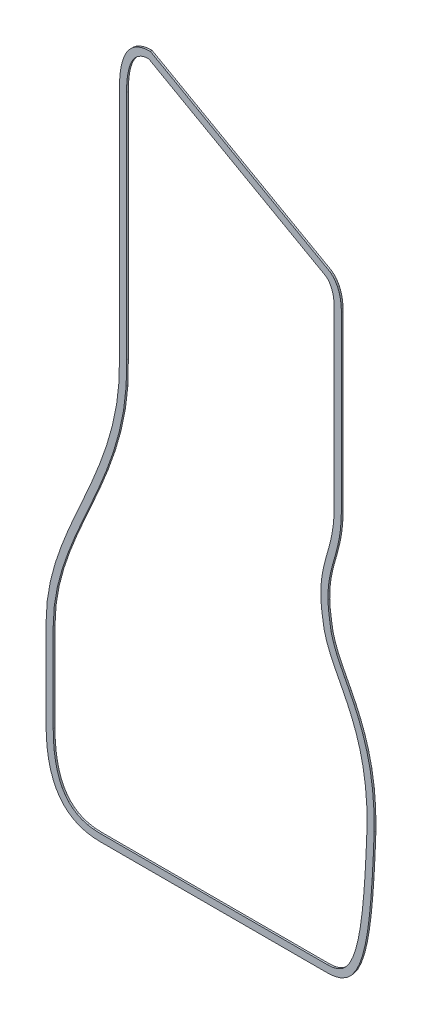
SolidWorks part; units mm, degrees
ref_plane "前视基准面" through (0, 0, 0) normal (0, 0, 1) x (1, 0, 0)
ref_plane "上视基准面" through (0, 0, 0) normal (0, 1, 0) x (1, 0, 0)
ref_plane "右视基准面" through (0, 0, 0) normal (1, 0, 0) x (0, 0, -1)
other "Configuration Table"
sketch "草图1" plane through (0, 0, 0) normal (0, 0, 1) x (1, 0, 0)
  line L0 (103, 235) -> (-24.8333, 235)
  line L1 (-24.8333, 235) -> (-152.6667, 235)
  line L2 (-152.6667, 235) -> (-280.5, 235)
  line L3 (-280.5, 235) -> (-293.0357, 235.6378)
  line L4 (-293.0357, 235.6378) -> (-304.6429, 237.551)
  line L5 (-304.6429, 237.551) -> (-315.3214, 240.7398)
  line L6 (-315.3214, 240.7398) -> (-325.0714, 245.2041)
  line L7 (-325.0714, 245.2041) -> (-333.8929, 250.9439)
  line L8 (-333.8929, 250.9439) -> (-341.7857, 257.9592)
  line L9 (-341.7857, 257.9592) -> (-348.75, 266.25)
  line L10 (-348.75, 266.25) -> (-354.7857, 275.8163)
  line L11 (-354.7857, 275.8163) -> (-359.8929, 286.6582)
  line L12 (-359.8929, 286.6582) -> (-364.0714, 298.7755)
  line L13 (-364.0714, 298.7755) -> (-367.3214, 312.1684)
  line L14 (-367.3214, 312.1684) -> (-369.6429, 326.8367)
  line L15 (-369.6429, 326.8367) -> (-371.0357, 342.7806)
  line L16 (-371.0357, 342.7806) -> (-371.5, 360)
  line L17 (-371.5, 360) -> (-371.5, 410)
  line L18 (-371.5, 410) -> (-371.5, 460)
  line L19 (-371.5, 460) -> (-371.5, 510)
  line L20 (-371.5, 510) -> (-369.6073, 541.7165)
  line L21 (-369.6073, 541.7165) -> (-364.3178, 572.7114)
  line L22 (-364.3178, 572.7114) -> (-356.2141, 603.1815)
  line L23 (-356.2141, 603.1815) -> (-345.879, 633.3236)
  line L24 (-345.879, 633.3236) -> (-333.8952, 663.3345)
  line L25 (-333.8952, 663.3345) -> (-320.8455, 693.4111)
  line L26 (-320.8455, 693.4111) -> (-307.3125, 723.75)
  line L27 (-307.3125, 723.75) -> (-293.879, 754.5481)
  line L28 (-293.879, 754.5481) -> (-281.1277, 786.0022)
  line L29 (-281.1277, 786.0022) -> (-269.6414, 818.309)
  line L30 (-269.6414, 818.309) -> (-260.0027, 851.6655)
  line L31 (-260.0027, 851.6655) -> (-252.7945, 886.2682)
  line L32 (-252.7945, 886.2682) -> (-248.5993, 922.3141)
  line L33 (-248.5993, 922.3141) -> (-248, 960)
  line L34 (-248, 960) -> (-248, 1090)
  line L35 (-248, 1090) -> (-248, 1220)
  line L36 (-248, 1220) -> (-248, 1350)
  line L37 (-248, 1350) -> (-247.7347, 1361.0204)
  line L38 (-247.7347, 1361.0204) -> (-246.9388, 1371.2245)
  line L39 (-246.9388, 1371.2245) -> (-245.6122, 1380.6122)
  line L40 (-245.6122, 1380.6122) -> (-243.7551, 1389.1837)
  line L41 (-243.7551, 1389.1837) -> (-241.3673, 1396.9388)
  line L42 (-241.3673, 1396.9388) -> (-238.449, 1403.8776)
  line L43 (-238.449, 1403.8776) -> (-235, 1410)
  line L44 (-235, 1410) -> (-231.0204, 1415.3061)
  line L45 (-231.0204, 1415.3061) -> (-226.5102, 1419.7959)
  line L46 (-226.5102, 1419.7959) -> (-221.4694, 1423.4694)
  line L47 (-221.4694, 1423.4694) -> (-215.898, 1426.3265)
  line L48 (-215.898, 1426.3265) -> (-209.7959, 1428.3673)
  line L49 (-209.7959, 1428.3673) -> (-203.1633, 1429.5918)
  line L50 (-203.1633, 1429.5918) -> (-196, 1430)
  line L51 (-196, 1430) -> (-95.25, 1373.3333)
  line L52 (-95.25, 1373.3333) -> (5.5, 1316.6667)
  line L53 (5.5, 1316.6667) -> (106.25, 1260)
  line L54 (106.25, 1260) -> (108.9362, 1257.8878)
  line L55 (108.9362, 1257.8878) -> (111.4235, 1255.551)
  line L56 (111.4235, 1255.551) -> (113.7117, 1252.9898)
  line L57 (113.7117, 1252.9898) -> (115.801, 1250.2041)
  line L58 (115.801, 1250.2041) -> (117.6913, 1247.1939)
  line L59 (117.6913, 1247.1939) -> (119.3827, 1243.9592)
  line L60 (119.3827, 1243.9592) -> (120.875, 1240.5)
  line L61 (120.875, 1240.5) -> (122.1684, 1236.8163)
  line L62 (122.1684, 1236.8163) -> (123.2628, 1232.9082)
  line L63 (123.2628, 1232.9082) -> (124.1582, 1228.7755)
  line L64 (124.1582, 1228.7755) -> (124.8546, 1224.4184)
  line L65 (124.8546, 1224.4184) -> (125.352, 1219.8367)
  line L66 (125.352, 1219.8367) -> (125.6505, 1215.0306)
  line L67 (125.6505, 1215.0306) -> (125.75, 1210)
  line L68 (125.75, 1210) -> (125.75, 1113.3333)
  line L69 (125.75, 1113.3333) -> (125.75, 1016.6667)
  line L70 (125.75, 1016.6667) -> (125.75, 920)
  line L71 (125.75, 920) -> (125.281, 904.7303)
  line L72 (125.281, 904.7303) -> (123.9876, 890.9038)
  line L73 (123.9876, 890.9038) -> (122.0405, 878.2799)
  line L74 (122.0405, 878.2799) -> (119.6101, 866.6181)
  line L75 (119.6101, 866.6181) -> (116.867, 855.6778)
  line L76 (116.867, 855.6778) -> (113.9818, 845.2187)
  line L77 (113.9818, 845.2187) -> (111.125, 835)
  line L78 (111.125, 835) -> (108.4672, 824.7813)
  line L79 (108.4672, 824.7813) -> (106.1789, 814.3222)
  line L80 (106.1789, 814.3222) -> (104.4308, 803.3819)
  line L81 (104.4308, 803.3819) -> (103.3932, 791.7201)
  line L82 (103.3932, 791.7201) -> (103.2369, 779.0962)
  line L83 (103.2369, 779.0962) -> (104.1323, 765.2697)
  line L84 (104.1323, 765.2697) -> (106.25, 750)
  line L85 (106.25, 750) -> (108.5868, 735.4045)
  line L86 (108.5868, 735.4045) -> (112.6079, 721.3994)
  line L87 (112.6079, 721.3994) -> (118.0076, 707.6567)
  line L88 (118.0076, 707.6567) -> (124.4803, 693.8484)
  line L89 (124.4803, 693.8484) -> (131.7206, 679.6465)
  line L90 (131.7206, 679.6465) -> (139.4227, 664.723)
  line L91 (139.4227, 664.723) -> (147.2812, 648.75)
  line L92 (147.2812, 648.75) -> (154.9905, 631.3994)
  line L93 (154.9905, 631.3994) -> (162.245, 612.3433)
  line L94 (162.245, 612.3433) -> (168.7391, 591.2536)
  line L95 (168.7391, 591.2536) -> (174.1672, 567.8025)
  line L96 (174.1672, 567.8025) -> (178.2238, 541.6618)
  line L97 (178.2238, 541.6618) -> (180.6032, 512.5036)
  line L98 (180.6032, 512.5036) -> (181, 480)
  line L99 (181, 480) -> (179.4934, 443.1706)
  line L100 (179.4934, 443.1706) -> (177.7026, 409.7522)
  line L101 (177.7026, 409.7522) -> (175.5423, 379.6356)
  line L102 (175.5423, 379.6356) -> (172.9271, 352.7114)
  line L103 (172.9271, 352.7114) -> (169.7719, 328.8703)
  line L104 (169.7719, 328.8703) -> (165.9913, 308.0029)
  line L105 (165.9913, 308.0029) -> (161.5, 290)
  line L106 (161.5, 290) -> (156.2128, 274.7522)
  line L107 (156.2128, 274.7522) -> (150.0445, 262.1501)
  line L108 (150.0445, 262.1501) -> (142.9096, 252.0845)
  line L109 (142.9096, 252.0845) -> (134.723, 244.4461)
  line L110 (134.723, 244.4461) -> (125.3994, 239.1254)
  line L111 (125.3994, 239.1254) -> (114.8535, 236.0131)
  line L112 (114.8535, 236.0131) -> (103, 235)
  line L113 (102.4881, 247) -> (-280.1949, 247)
  line L114 (-280.1949, 247) -> (-291.751, 247.5879)
  line L115 (-291.751, 247.5879) -> (-301.9394, 249.2673)
  line L116 (-301.9394, 249.2673) -> (-311.0863, 251.9987)
  line L117 (-311.0863, 251.9987) -> (-319.2698, 255.7457)
  line L118 (-319.2698, 255.7457) -> (-326.5937, 260.5112)
  line L119 (-326.5937, 260.5112) -> (-333.1599, 266.3473)
  line L120 (-333.1599, 266.3473) -> (-339.0366, 273.3434)
  line L121 (-339.0366, 273.3434) -> (-344.2438, 281.5965)
  line L122 (-344.2438, 281.5965) -> (-348.7602, 291.1843)
  line L123 (-348.7602, 291.1843) -> (-352.543, 302.1539)
  line L124 (-352.543, 302.1539) -> (-355.5451, 314.5251)
  line L125 (-355.5451, 314.5251) -> (-357.7249, 328.2986)
  line L126 (-357.7249, 328.2986) -> (-359.0498, 343.4651)
  line L127 (-359.0498, 343.4651) -> (-359.5, 360.1617)
  line L128 (-359.5, 360.1617) -> (-359.5, 509.6423)
  line L129 (-359.5, 509.6423) -> (-357.6678, 540.3456)
  line L130 (-357.6678, 540.3456) -> (-352.5806, 570.1546)
  line L131 (-352.5806, 570.1546) -> (-344.7258, 599.689)
  line L132 (-344.7258, 599.689) -> (-334.6243, 629.1499)
  line L133 (-334.6243, 629.1499) -> (-322.8164, 658.7203)
  line L134 (-322.8164, 658.7203) -> (-309.8614, 688.5785)
  line L135 (-309.8614, 688.5785) -> (-296.3533, 718.8616)
  line L136 (-296.3533, 718.8616) -> (-296.3133, 718.9524)
  line L137 (-296.3133, 718.9524) -> (-282.8798, 749.7505)
  line L138 (-282.8798, 749.7505) -> (-282.7581, 750.0398)
  line L139 (-282.7581, 750.0398) -> (-270.0068, 781.4938)
  line L140 (-270.0068, 781.4938) -> (-269.8211, 781.9822)
  line L141 (-269.8211, 781.9822) -> (-258.3348, 814.2891)
  line L142 (-258.3348, 814.2891) -> (-258.113, 814.9778)
  line L143 (-258.113, 814.9778) -> (-248.4744, 848.3342)
  line L144 (-248.4744, 848.3342) -> (-248.2549, 849.2182)
  line L145 (-248.2549, 849.2182) -> (-241.0467, 883.821)
  line L146 (-241.0467, 883.821) -> (-240.8749, 884.881)
  line L147 (-240.8749, 884.881) -> (-236.6798, 920.9269)
  line L148 (-236.6798, 920.9269) -> (-236.6008, 922.1233)
  line L149 (-236.6008, 922.1233) -> (-236.0015, 959.8092)
  line L150 (-236.0015, 959.8092) -> (-236, 960)
  line L151 (-236, 960) -> (-236, 1349.8556)
  line L152 (-236, 1349.8556) -> (-235.7459, 1360.409)
  line L153 (-235.7459, 1360.409) -> (-235.0043, 1369.9171)
  line L154 (-235.0043, 1369.9171) -> (-233.7916, 1378.4994)
  line L155 (-233.7916, 1378.4994) -> (-232.1357, 1386.142)
  line L156 (-232.1357, 1386.142) -> (-230.0744, 1392.8369)
  line L157 (-230.0744, 1392.8369) -> (-227.6551, 1398.5891)
  line L158 (-227.6551, 1398.5891) -> (-224.9296, 1403.4272)
  line L159 (-224.9296, 1403.4272) -> (-221.9403, 1407.4129)
  line L160 (-221.9403, 1407.4129) -> (-218.6976, 1410.6409)
  line L161 (-218.6976, 1410.6409) -> (-215.1595, 1413.2193)
  line L162 (-215.1595, 1413.2193) -> (-211.2304, 1415.2342)
  line L163 (-211.2304, 1415.2342) -> (-206.7888, 1416.7197)
  line L164 (-206.7888, 1416.7197) -> (-201.727, 1417.6542)
  line L165 (-201.727, 1417.6542) -> (-198.8226, 1417.8197)
  line L166 (-198.8226, 1417.8197) -> (-101.1327, 1362.8742)
  line L167 (-101.1327, 1362.8742) -> (99.5603, 1249.9947)
  line L168 (99.5603, 1249.9947) -> (101.1041, 1248.7808)
  line L169 (101.1041, 1248.7808) -> (102.8244, 1247.1646)
  line L170 (102.8244, 1247.1646) -> (104.4203, 1245.3783)
  line L171 (104.4203, 1245.3783) -> (105.9029, 1243.4016)
  line L172 (105.9029, 1243.4016) -> (107.2769, 1241.2136)
  line L173 (107.2769, 1241.2136) -> (108.5414, 1238.7952)
  line L174 (108.5414, 1238.7952) -> (109.6911, 1236.1303)
  line L175 (109.6911, 1236.1303) -> (110.7175, 1233.2069)
  line L176 (110.7175, 1233.2069) -> (111.6107, 1230.0172)
  line L177 (111.6107, 1230.0172) -> (112.3606, 1226.5563)
  line L178 (112.3606, 1226.5563) -> (112.9573, 1222.8227)
  line L179 (112.9573, 1222.8227) -> (113.3923, 1218.8167)
  line L180 (113.3923, 1218.8167) -> (113.6579, 1214.5399)
  line L181 (113.6579, 1214.5399) -> (113.75, 1209.8814)
  line L182 (113.75, 1209.8814) -> (113.75, 920.1843)
  line L183 (113.75, 920.1843) -> (113.2982, 905.4741)
  line L184 (113.2982, 905.4741) -> (112.0732, 892.3786)
  line L185 (112.0732, 892.3786) -> (110.2287, 880.4201)
  line L186 (110.2287, 880.4201) -> (107.9117, 869.3025)
  line L187 (107.9117, 869.3025) -> (105.2616, 858.733)
  line L188 (105.2616, 858.733) -> (102.4193, 848.4296)
  line L189 (102.4193, 848.4296) -> (99.5681, 838.2309)
  line L190 (99.5681, 838.2309) -> (99.5114, 838.0206)
  line L191 (99.5114, 838.0206) -> (96.8536, 827.802)
  line L192 (96.8536, 827.802) -> (96.7445, 827.346)
  line L193 (96.7445, 827.346) -> (94.4562, 816.8869)
  line L194 (94.4562, 816.8869) -> (94.3293, 816.2157)
  line L195 (94.3293, 816.2157) -> (92.5811, 805.2754)
  line L196 (92.5811, 805.2754) -> (92.478, 804.4453)
  line L197 (92.478, 804.4453) -> (91.4404, 792.7835)
  line L198 (91.4404, 792.7835) -> (91.3941, 791.8687)
  line L199 (91.3941, 791.8687) -> (91.2378, 779.2448)
  line L200 (91.2378, 779.2448) -> (91.262, 778.3207)
  line L201 (91.262, 778.3207) -> (92.1574, 764.4942)
  line L202 (92.1574, 764.4942) -> (92.2461, 763.6212)
  line L203 (92.2461, 763.6212) -> (94.3638, 748.3515)
  line L204 (94.3638, 748.3515) -> (94.4009, 748.1029)
  line L205 (94.4009, 748.1029) -> (96.7377, 733.5074)
  line L206 (96.7377, 733.5074) -> (97.0528, 732.093)
  line L207 (97.0528, 732.093) -> (101.0739, 718.0879)
  line L208 (101.0739, 718.0879) -> (101.4391, 717.011)
  line L209 (101.4391, 717.011) -> (106.8388, 703.2683)
  line L210 (106.8388, 703.2683) -> (107.1421, 702.5634)
  line L211 (107.1421, 702.5634) -> (113.6148, 688.7551)
  line L212 (113.6148, 688.7551) -> (113.7895, 688.3981)
  line L213 (113.7895, 688.3981) -> (121.0297, 674.1962)
  line L214 (121.0297, 674.1962) -> (121.057, 674.1429)
  line L215 (121.057, 674.1429) -> (128.7063, 659.322)
  line L216 (128.7063, 659.322) -> (136.4103, 643.6631)
  line L217 (136.4103, 643.6631) -> (143.8918, 626.8251)
  line L218 (143.8918, 626.8251) -> (150.8913, 608.4387)
  line L219 (150.8913, 608.4387) -> (157.1446, 588.1309)
  line L220 (157.1446, 588.1309) -> (162.3768, 565.5263)
  line L221 (162.3768, 565.5263) -> (166.2989, 540.2519)
  line L222 (166.2989, 540.2519) -> (168.6092, 511.9417)
  line L223 (168.6092, 511.9417) -> (168.997, 480.1721)
  line L224 (168.997, 480.1721) -> (167.5066, 443.7369)
  line L225 (167.5066, 443.7369) -> (165.7256, 410.5026)
  line L226 (165.7256, 410.5026) -> (163.5839, 380.6451)
  line L227 (163.5839, 380.6451) -> (161.0035, 354.079)
  line L228 (161.0035, 354.079) -> (157.9131, 330.7282)
  line L229 (157.9131, 330.7282) -> (154.2533, 310.5276)
  line L230 (154.2533, 310.5276) -> (149.9866, 293.4248)
  line L231 (149.9866, 293.4248) -> (145.114, 279.3727)
  line L232 (145.114, 279.3727) -> (139.6931, 268.2977)
  line L233 (139.6931, 268.2977) -> (133.8278, 260.0231)
  line L234 (133.8278, 260.0231) -> (127.5598, 254.1747)
  line L235 (127.5598, 254.1747) -> (120.6641, 250.2395)
  line L236 (120.6641, 250.2395) -> (112.6216, 247.8661)
  line L237 (112.6216, 247.8661) -> (102.4881, 247)
  point P0 (0, 0)
  dimension "D1" = 0.4643
  dimension "D2" = 1.8571
  dimension "D3" = 1.8927
  dimension "D4" = 4.1786
  dimension "D5" = 7.1822
  dimension "D6" = 7.4286
  dimension "D7" = 11.6071
  dimension "D8" = 12
  dimension "D9" = 12.4502
  dimension "D10" = 13.7751
  dimension "D11" = 13.8322
  dimension "D12" = 15.2859
  dimension "D13" = 15.9549
  dimension "D14" = 16.7143
  dimension "D15" = 18.9194
  dimension "D16" = 18.957
  dimension "D17" = 22.7398
  dimension "D18" = 22.75
  dimension "D19" = 25.621
  dimension "D20" = 26.7742
  dimension "D21" = 27.2562
  dimension "D22" = 29.7143
  dimension "D23" = 32.4634
  dimension "D24" = 36.8757
  dimension "D25" = 37.6048
  dimension "D26" = 37.6071
  dimension "D27" = 38.3401
  dimension "D28" = 44.9063
  dimension "D29" = 46.4286
  dimension "D30" = 48.6836
  dimension "D31" = 50.6545
  dimension "D32" = 52.2302
  dimension "D33" = 56.1786
  dimension "D34" = 60.4137
  dimension "D35" = 61.6386
  dimension "D36" = 64.1875
  dimension "D37" = 66.8571
  dimension "D38" = 69.5606
  dimension "D39" = 75.1467
  dimension "D40" = 75.1867
  dimension "D41" = 77.621
  dimension "D42" = 78.4643
  dimension "D43" = 79.749
  dimension "D44" = 88.6202
  dimension "D45" = 88.7419
  dimension "D46" = 90.3723
  dimension "D47" = 91
  dimension "D48" = 91.3051
  dimension "D49" = 101.4932
  dimension "D50" = 101.6789
  dimension "D51" = 101.8586
  dimension "D52" = 111.4973
  dimension "D53" = 113.1652
  dimension "D54" = 113.387
  dimension "D55" = 118.7055
  dimension "D56" = 122.9007
  dimension "D57" = 123.0256
  dimension "D58" = 123.2451
  dimension "D59" = 123.5
  dimension "D60" = 123.7653
  dimension "D61" = 124.5612
  dimension "D62" = 125.8878
  dimension "D63" = 127.7449
  dimension "D64" = 130.1327
  dimension "D65" = 130.4533
  dimension "D66" = 130.6251
  dimension "D67" = 133.051
  dimension "D68" = 134.8202
  dimension "D69" = 134.8992
  dimension "D70" = 135.4985
  dimension "D71" = 135.5
  dimension "D72" = 135.7541
  dimension "D73" = 136.4957
  dimension "D74" = 136.5
  dimension "D75" = 137.7084
  dimension "D76" = 139.3643
  dimension "D77" = 140.4796
  dimension "D78" = 141.4256
  dimension "D79" = 143.8449
  dimension "D80" = 144.9898
  dimension "D81" = 146.5704
  dimension "D82" = 149.5597
  dimension "D83" = 150.0306
  dimension "D84" = 152.8024
  dimension "D85" = 155.602
  dimension "D86" = 156.3405
  dimension "D87" = 160.2696
  dimension "D88" = 161.7041
  dimension "D89" = 164.7112
  dimension "D90" = 168.3367
  dimension "D91" = 169.773
  dimension "D92" = 172.6774
  dimension "D93" = 175.5
  dimension "D94" = 218.8333
  dimension "D95" = 270.3673
  dimension "D96" = 276.25
  dimension "D97" = 346.6667
  dimension "D98" = 371.5
  dimension "D99" = 377
  dimension "D100" = 462.7378
  dimension "D101" = 462.762
  dimension "D102" = 462.8941
  dimension "D103" = 462.9404
  dimension "D104" = 463.6574
  dimension "D105" = 463.7461
  dimension "D106" = 463.978
  dimension "D107" = 464.0811
  dimension "D108" = 465.8293
  dimension "D109" = 465.8638
  dimension "D110" = 465.9009
  dimension "D111" = 465.9562
  dimension "D112" = 468.2377
  dimension "D113" = 468.2445
  dimension "D114" = 468.3536
  dimension "D115" = 468.5528
  dimension "D116" = 471.0114
  dimension "D117" = 471.0603
  dimension "D118" = 471.0681
  dimension "D119" = 472.5739
  dimension "D120" = 472.6041
  dimension "D121" = 472.9391
  dimension "D122" = 473.9193
  dimension "D123" = 473.9881
  dimension "D124" = 474.3244
  dimension "D125" = 474.5
  dimension "D126" = 474.7369
  dimension "D127" = 474.8932
  dimension "D128" = 475.6323
  dimension "D129" = 475.9203
  dimension "D130" = 475.9308
  dimension "D131" = 476.7616
  dimension "D132" = 477.4029
  dimension "D133" = 477.6789
  dimension "D134" = 477.75
  dimension "D135" = 478.3388
  dimension "D136" = 478.6421
  dimension "D137" = 478.7769
  dimension "D138" = 479.4117
  dimension "D139" = 479.9672
  dimension "D140" = 480.0414
  dimension "D141" = 480.0868
  dimension "D142" = 480.4362
  dimension "D143" = 481.1911
  dimension "D144" = 481.7287
  dimension "D145" = 482.2175
  dimension "D146" = 482.625
  dimension "D147" = 482.9235
  dimension "D148" = 483.1107
  dimension "D149" = 483.5732
  dimension "D150" = 483.8606
  dimension "D151" = 484.1079
  dimension "D152" = 484.1216
  dimension "D153" = 484.4573
  dimension "D154" = 484.7982
  dimension "D155" = 484.8923
  dimension "D156" = 485.1148
  dimension "D157" = 485.1579
  dimension "D158" = 485.2117
  dimension "D159" = 485.25
  dimension "D160" = 485.2895
  dimension "D161" = 485.4818
  dimension "D162" = 486.3535
  dimension "D163" = 487.301
  dimension "D164" = 488.367
  dimension "D165" = 489.1913
  dimension "D166" = 489.5076
  dimension "D167" = 490.8827
  dimension "D168" = 491.1101
  dimension "D169" = 492.1641
  dimension "D170" = 492.375
  dimension "D171" = 492.5297
  dimension "D172" = 492.557
  dimension "D173" = 493.5405
  dimension "D174" = 493.6684
  dimension "D175" = 494.7628
  dimension "D176" = 495.4876
  dimension "D177" = 495.6582
  dimension "D178" = 495.9803
  dimension "D179" = 496.3546
  dimension "D180" = 496.781
  dimension "D181" = 496.852
  dimension "D182" = 496.8994
  dimension "D183" = 497.1505
  dimension "D184" = 497.25
  dimension "D185" = 499.0598
  dimension "D186" = 500.2063
  dimension "D187" = 503.2206
  dimension "D188" = 505.3278
  dimension "D189" = 506.223
  dimension "D190" = 507.9103
  dimension "D191" = 510.9227
  dimension "D192" = 511.1931
  dimension "D193" = 514.4096
  dimension "D194" = 515.3918
  dimension "D195" = 516.614
  dimension "D196" = 518.7812
  dimension "D197" = 521.4866
  dimension "D198" = 521.5445
  dimension "D199" = 522.3913
  dimension "D200" = 525.7533
  dimension "D201" = 526.4905
  dimension "D202" = 527.7128
  dimension "D203" = 528.6446
  dimension "D204" = 529.4131
  dimension "D205" = 532.5035
  dimension "D206" = 533
  dimension "D207" = 533.745
  dimension "D208" = 533.8768
  dimension "D209" = 535.0839
  dimension "D210" = 537.2256
  dimension "D211" = 537.4913
  dimension "D212" = 537.7989
  dimension "D213" = 539.0066
  dimension "D214" = 540.1092
  dimension "D215" = 540.2391
  dimension "D216" = 540.497
  dimension "D217" = 541.2719
  dimension "D218" = 544.4271
  dimension "D219" = 545.6672
  dimension "D220" = 547.0423
  dimension "D221" = 549.2026
  dimension "D222" = 549.7238
  dimension "D223" = 550.9934
  dimension "D224" = 552.1032
  dimension "D225" = 552.5
  dimension "D226" = 0.6378
  dimension "D227" = 1.0131
  dimension "D228" = 2.551
  dimension "D229" = 4.1254
  dimension "D230" = 5.7398
  dimension "D231" = 9.4461
  dimension "D232" = 10.2041
  dimension "D233" = 12
  dimension "D234" = 12.5879
  dimension "D235" = 12.8661
  dimension "D236" = 14.2673
  dimension "D237" = 15.2395
  dimension "D238" = 15.9439
  dimension "D239" = 16.9987
  dimension "D240" = 17.0845
  dimension "D241" = 19.1747
  dimension "D242" = 20.7457
  dimension "D243" = 22.9592
  dimension "D244" = 25.0231
  dimension "D245" = 25.5112
  dimension "D246" = 27.1501
  dimension "D247" = 31.25
  dimension "D248" = 31.3473
  dimension "D249" = 33.2977
  dimension "D250" = 38.3434
  dimension "D251" = 39.7522
  dimension "D252" = 40.8163
  dimension "D253" = 44.3727
  dimension "D254" = 46.5965
  dimension "D255" = 51.6582
  dimension "D256" = 55
  dimension "D257" = 56.1843
  dimension "D258" = 58.4248
  dimension "D259" = 63.7755
  dimension "D260" = 67.1539
  dimension "D261" = 73.0029
  dimension "D262" = 75.5276
  dimension "D263" = 77.1684
  dimension "D264" = 79.5251
  dimension "D265" = 91.8367
  dimension "D266" = 93.2986
  dimension "D267" = 93.8703
  dimension "D268" = 95.7282
  dimension "D269" = 107.7806
  dimension "D270" = 108.4651
  dimension "D271" = 117.7114
  dimension "D272" = 119.079
  dimension "D273" = 125
  dimension "D274" = 125.1617
  dimension "D275" = 144.6356
  dimension "D276" = 145.6451
  dimension "D277" = 174.7522
  dimension "D278" = 175
  dimension "D279" = 175.5026
  dimension "D280" = 208.1706
  dimension "D281" = 208.7369
  dimension "D282" = 225
  dimension "D283" = 245
  dimension "D284" = 245.1721
  dimension "D285" = 274.6423
  dimension "D286" = 275
  dimension "D287" = 276.9417
  dimension "D288" = 277.5036
  dimension "D289" = 305.2519
  dimension "D290" = 305.3456
  dimension "D291" = 306.6618
  dimension "D292" = 306.7165
  dimension "D293" = 330.5263
  dimension "D294" = 332.8025
  dimension "D295" = 335.1546
  dimension "D296" = 337.7114
  dimension "D297" = 353.1309
  dimension "D298" = 356.2536
  dimension "D299" = 364.689
  dimension "D300" = 368.1815
  dimension "D301" = 373.4387
  dimension "D302" = 377.3433
  dimension "D303" = 391.8251
  dimension "D304" = 394.1499
  dimension "D305" = 396.3994
  dimension "D306" = 398.3236
  dimension "D307" = 408.6631
  dimension "D308" = 413.75
  dimension "D309" = 423.7203
  dimension "D310" = 424.322
  dimension "D311" = 428.3345
  dimension "D312" = 429.723
  dimension "D313" = 439.1429
  dimension "D314" = 439.1962
  dimension "D315" = 444.6465
  dimension "D316" = 453.3981
  dimension "D317" = 453.5785
  dimension "D318" = 453.7551
  dimension "D319" = 458.4111
  dimension "D320" = 458.8484
  dimension "D321" = 467.5634
  dimension "D322" = 468.2683
  dimension "D323" = 472.6567
  dimension "D324" = 482.011
  dimension "D325" = 483.0879
  dimension "D326" = 483.8616
  dimension "D327" = 483.9524
  dimension "D328" = 486.3994
  dimension "D329" = 488.75
  dimension "D330" = 497.093
  dimension "D331" = 498.5074
  dimension "D332" = 500.4045
  dimension "D333" = 513.1029
  dimension "D334" = 513.3515
  dimension "D335" = 514.7505
  dimension "D336" = 515
  dimension "D337" = 515.0398
  dimension "D338" = 519.5481
  dimension "D339" = 528.6212
  dimension "D340" = 529.4942
  dimension "D341" = 530.2697
  dimension "D342" = 543.3207
  dimension "D343" = 544.0962
  dimension "D344" = 544.2448
  dimension "D345" = 546.4938
  dimension "D346" = 546.9822
  dimension "D347" = 551.0022
  dimension "D348" = 556.7201
  dimension "D349" = 556.8687
  dimension "D350" = 557.7835
  dimension "D351" = 568.3819
  dimension "D352" = 569.4453
  dimension "D353" = 570.2754
  dimension "D354" = 579.2891
  dimension "D355" = 579.3222
  dimension "D356" = 579.9778
  dimension "D357" = 581.2157
  dimension "D358" = 581.8869
  dimension "D359" = 583.309
  dimension "D360" = 589.7813
  dimension "D361" = 592.346
  dimension "D362" = 592.802
  dimension "D363" = 600
  dimension "D364" = 603.0206
  dimension "D365" = 603.2309
  dimension "D366" = 610.2187
  dimension "D367" = 613.3342
  dimension "D368" = 613.4296
  dimension "D369" = 614.2182
  dimension "D370" = 616.6655
  dimension "D371" = 620.6778
  dimension "D372" = 623.733
  dimension "D373" = 631.6181
  dimension "D374" = 634.3025
  dimension "D375" = 643.2799
  dimension "D376" = 645.4201
  dimension "D377" = 648.821
  dimension "D378" = 649.881
  dimension "D379" = 651.2682
  dimension "D380" = 655.9038
  dimension "D381" = 657.3786
  dimension "D382" = 669.7303
  dimension "D383" = 670.4741
  dimension "D384" = 685
  dimension "D385" = 685.1843
  dimension "D386" = 685.9269
  dimension "D387" = 687.1233
  dimension "D388" = 687.3141
  dimension "D389" = 724.8092
  dimension "D390" = 725
  dimension "D391" = 781.6667
  dimension "D392" = 855
  dimension "D393" = 878.3333
  dimension "D394" = 974.8814
  dimension "D395" = 975
  dimension "D396" = 979.5399
  dimension "D397" = 980.0306
  dimension "D398" = 983.8167
  dimension "D399" = 984.8367
  dimension "D400" = 985
  dimension "D401" = 987.8227
  dimension "D402" = 989.4184
  dimension "D403" = 991.5563
  dimension "D404" = 993.7755
  dimension "D405" = 995.0172
  dimension "D406" = 997.9082
  dimension "D407" = 998.2069
  dimension "D408" = 1001.1303
  dimension "D409" = 1001.8163
  dimension "D410" = 1003.7952
  dimension "D411" = 1005.5
  dimension "D412" = 1006.2136
  dimension "D413" = 1008.4016
  dimension "D414" = 1008.9592
  dimension "D415" = 1010.3783
  dimension "D416" = 1012.1646
  dimension "D417" = 1012.1939
  dimension "D418" = 1013.7808
  dimension "D419" = 1014.9947
  dimension "D420" = 1015.2041
  dimension "D421" = 1017.9898
  dimension "D422" = 1020.551
  dimension "D423" = 1022.8878
  dimension "D424" = 1025
  dimension "D425" = 1081.6667
  dimension "D426" = 1114.8556
  dimension "D427" = 1115
  dimension "D428" = 1125.409
  dimension "D429" = 1126.0204
  dimension "D430" = 1127.8742
  dimension "D431" = 1134.9171
  dimension "D432" = 1136.2245
  dimension "D433" = 235
  dimension "D434" = 1143.4994
  dimension "D435" = 1145.6122
  dimension "D436" = 1151.142
  dimension "D437" = 1154.1837
  dimension "D438" = 1157.8369
  dimension "D439" = 1161.9388
  dimension "D440" = 1163.5891
  dimension "D441" = 1168.4272
  dimension "D442" = 1168.8776
  dimension "D443" = 1172.4129
  dimension "D444" = 1175
  dimension "D445" = 1175.6409
  dimension "D446" = 1178.2193
  dimension "D447" = 1180.2342
  dimension "D448" = 1180.3061
  dimension "D449" = 1181.7197
  dimension "D450" = 1182.6542
  dimension "D452" = 1184.7959
  dimension "D453" = 1188.4694
  dimension "D454" = 1191.3265
  dimension "D455" = 1193.3673
  dimension "D456" = 1194.5918
extrude "凸台-拉伸1" add sketch "草图1" against normal mid plane 3
